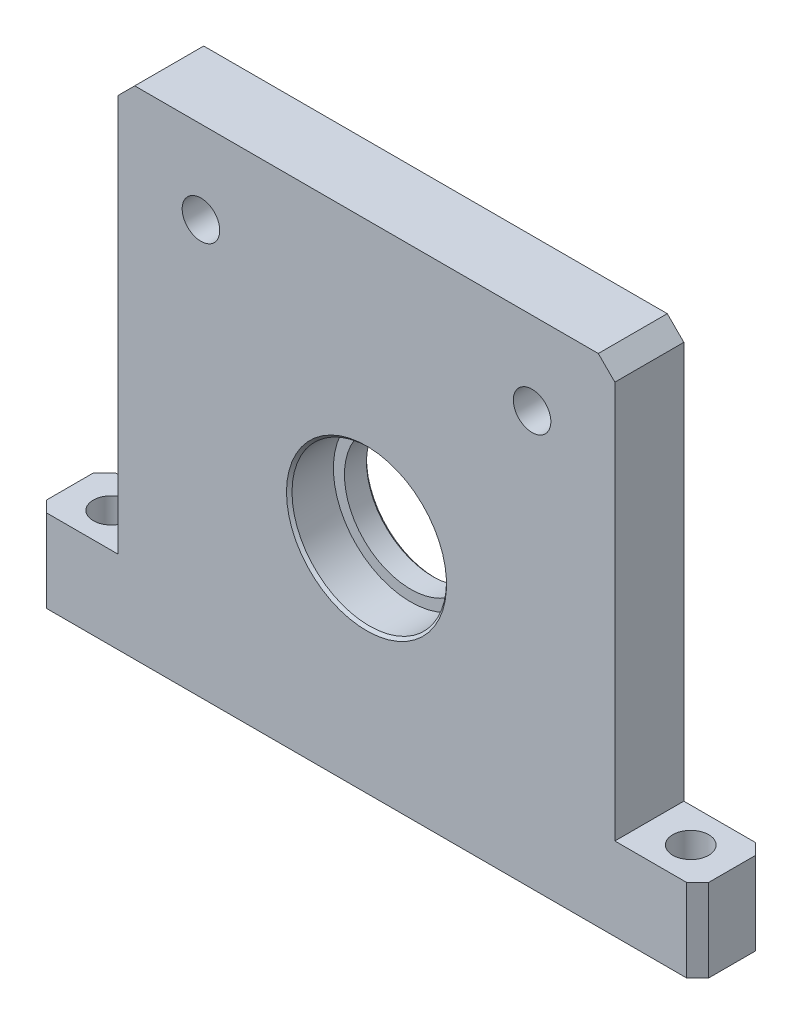
SolidWorks part; units mm, degrees
material "A6061"
ref_plane "Front" through (0, 0, 0) normal (0, 0, 1) x (1, 0, 0)
ref_plane "Top" through (0, 0, 0) normal (0, 1, 0) x (1, 0, 0)
ref_plane "Right" through (0, 0, 0) normal (1, 0, 0) x (0, 0, -1)
sketch "草图1" plane through (0, 0, 0) normal (1, 0, 0) x (0, 0, -1)
  line L0 (0, 0) -> (0, 90)
  line L1 (0, 90) -> (12.5, 90)
  line L2 (12.5, 90) -> (12.5, 0)
  line L5 (12.5, 0) -> (0, 0)
  dimension "D1" = 90
  dimension "D2" = 12.5
extrude "凸台-拉伸1" add sketch "草图1" along normal blind 90
chamfer "倒角1" distance 3 angle 45 2 edges at (0, 90, -6.25) (90, 90, -6.25)
hole_wizard "M8 螺纹孔1" positions "草图5" profile "草图4" tap size "M8" standard "Gb" end condition through all
sketch "草图5" plane through (0, 0, -12.5) normal (0, 0, -1) x (-1, 0, 0)
  line L4 (-90, 0) -> (0, 0) construction
  line L5 (-45, 0) -> (-45, 90) construction
  line L6 (-87, 90) -> (-3, 90) construction
  point P0 (-15, 75)
  point P2 (-75, 75)
  dimension "D2" = 75
  dimension "D3" = 60
cosmetic thread "孔螺蚊线1" parameters "D2"=8
cosmetic thread "孔螺蚊线2" parameters "D2"=8
sketch "草图4" plane through (15, 75, -12.5) normal (1, 0, 0) x (0, 1, 0)
  line L0 (0, 0) -> (0, 12.5)
  line L1 (0, 12.5) -> (3.4, 12.5)
  line L2 (3.4, 12.5) -> (3.4, 0)
  line L5 (3.4, 0) -> (0, 0)
  line L11 (0, -6.35) -> (0, 107.95) construction
  dimension "通孔螺纹孔钻头直径" = 6.8
  dimension "通孔螺纹孔钻头深度" = 12.5
sketch "草图6" plane through (0, 0, 0) normal (0, 0, 1) x (1, 0, 0)
  line L1 (0, 87) -> (0, 0) construction
  line L2 (90, 0) -> (0, 0) construction
  circle A0 centre (45, 40) radius 14
  dimension "D1" = 28
  dimension "D2" = 40
  dimension "D3" = 45
extrude "切除-拉伸1" cut sketch "草图6" against normal blind 8
sketch "草图7" plane through (0, 0, -8) normal (0, 0, 1) x (1, 0, 0)
  circle A0 centre (45, 40) radius 12
  dimension "D1" = 24
extrude "切除-拉伸2" cut sketch "草图7" against normal through all
chamfer "倒角2" distance 0.5 angle 45 2 edges at (57, 40, -12.5) (59, 40, 0)
sketch "草图10" plane through (90, 0, 0) normal (1, 0, 0) x (0, 0, -1)
  line L0 (12.5, 0) -> (12.5, 87) construction
  line L1 (0, 0) -> (12.5, 0)
  line L2 (0, 0) -> (0, 15)
  line L3 (0, 15) -> (12.5, 15)
  line L4 (12.5, 0) -> (12.5, 15)
  dimension "D1" = 15
extrude "凸台-拉伸3" add sketch "草图10" along normal blind 15
sketch "草图11" plane through (0, 0, 0) normal (-1, 0, 0) x (0, 0, 1)
  line L0 (-12.5, 0) -> (-12.5, 87) construction
  line L1 (-12.5, 15) -> (0, 15)
  line L2 (-12.5, 15) -> (-12.5, 0)
  line L3 (-12.5, 0) -> (0, 0)
  line L4 (0, 15) -> (0, 0)
  dimension "D1" = 15
extrude "凸台-拉伸4" add sketch "草图11" along normal blind 15
chamfer "倒角4" distance 2 angle 45 4 edges at (105, 7.5, 0) (-15, 7.5, 0) (-15, 7.5, -12.5) (105, 7.5, -12.5)
hole_wizard "Ø6.5 (6.5) 直径孔1" positions "草图13" profile "草图12" hole size "Ø6.5" standard "Iso" end condition through all
sketch "草图13" plane through (-61.7581, 15, 1.95) normal (0, 1, 0) x (1, 0, 0)
  line L4 (106.7581, 14.45) -> (106.7581, 1.95) construction
  line L7 (48.7581, 1.95) -> (61.7581, 1.95) construction
  line L8 (148.7581, 1.95) -> (64.7581, 1.95) construction
  line L9 (148.7581, 14.45) -> (64.7581, 14.45) construction
  point P0 (159.2581, 8.2)
  point P2 (54.2581, 8.2)
  dimension "D1" = 105
  dimension "D2" = 6.25
sketch "草图12" plane through (97.5, 15, -6.25) normal (1, 0, 0) x (0, 0, 1)
  line L0 (0, 0) -> (0, 15)
  line L1 (0, 15) -> (3.25, 15)
  line L2 (3.25, 15) -> (3.25, 0)
  line L5 (3.25, 0) -> (0, 0)
  line L11 (0, -6.35) -> (0, 107.95) construction
  dimension "通孔孔直径" = 6.5
  dimension "通孔孔深度" = 15
